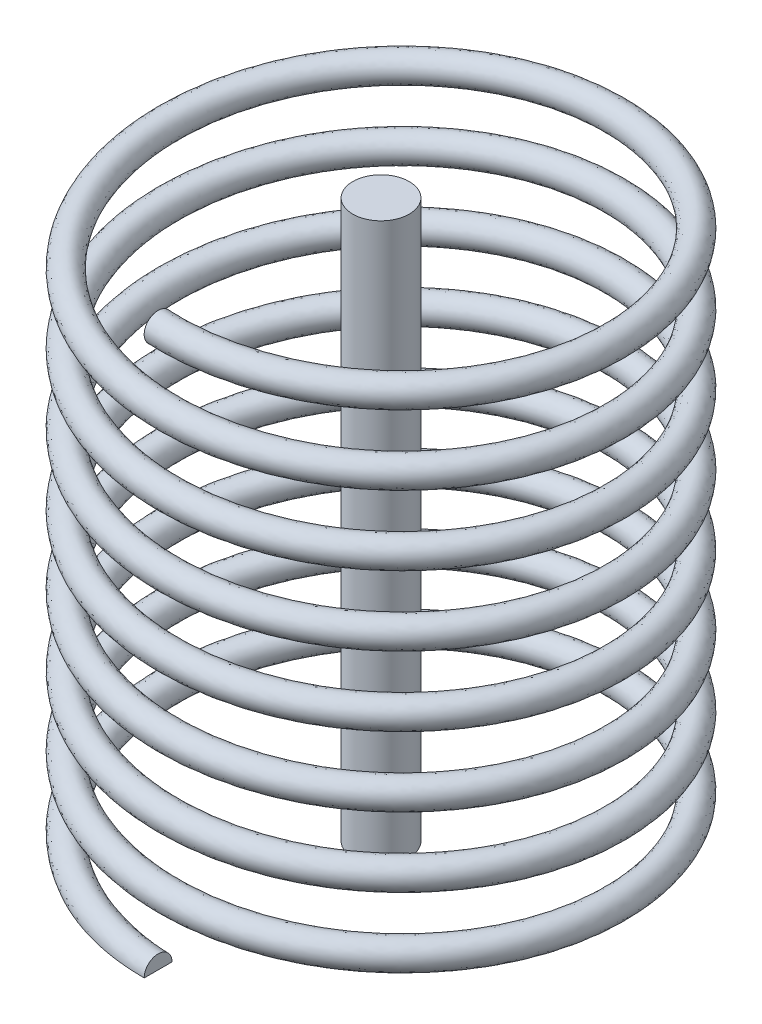
SolidWorks part; units mm, degrees
ref_plane "前视" through (0, 0, 0) normal (0, 0, 1) x (1, 0, 0)
ref_plane "上视" through (0, 0, 0) normal (0, 1, 0) x (1, 0, 0)
ref_plane "右视" through (0, 0, 0) normal (1, 0, 0) x (0, 0, -1)
sketch "草图2" plane through (0, 0, 0) normal (0, 1, 0) x (1, 0, 0)
  circle A0 centre (0, 0) radius 4
  dimension "D1" = 8
curve "螺旋线/涡状线1" pitch 1.25 height 10 turns 8
sketch "草图3" plane through (0, 0, 0) normal (1, 0, 0) x (0, 0, -1)
  line L0 (0, 0) -> (-4, 0) construction
  circle A0 centre (-4, 0) radius 0.25
  spline S0 degree 3 poles (-4, 0) (-4, 0.0259) (-3.7917, 0.0782) (-2.9021, 0.1562) (-1.5706, 0.2344) (0, 0.3125) (1.5706, 0.3906) (2.9021, 0.4687) (3.7917, 0.5469) (4.1041, 0.625) (3.7917, 0.7031) (2.9021, 0.7812) (1.5706, 0.8594) (0, 0.9375) (-1.5706, 1.0156) (-2.9021, 1.0937) (-3.7917, 1.1719) (-4.1041, 1.25) (-3.7917, 1.3281) (-2.9021, 1.4062) (-1.5706, 1.4844) (0, 1.5625) (1.5706, 1.6406) (2.9021, 1.7188) (3.7917, 1.7969) (4.1041, 1.875) (3.7917, 1.9531) (2.9021, 2.0313) (1.5706, 2.1094) (0, 2.1875) (-1.5706, 2.2656) (-2.9021, 2.3438) (-3.7917, 2.4219) (-4.1041, 2.5) (-3.7917, 2.5781) (-2.9021, 2.6562) (-1.5706, 2.7344) (0, 2.8125) (1.5706, 2.8906) (2.9021, 2.9688) (3.7917, 3.0469) (4.1041, 3.125) (3.7917, 3.2031) (2.9021, 3.2813) (1.5706, 3.3594) (0, 3.4375) (-1.5706, 3.5156) (-2.9021, 3.5938) (-3.7917, 3.6719) (-4.1041, 3.75) (-3.7917, 3.8281) (-2.9021, 3.9063) (-1.5706, 3.9844) (0, 4.0625) (1.5706, 4.1406) (2.9021, 4.2188) (3.7917, 4.2969) (4.1041, 4.375) (3.7917, 4.4531) (2.9021, 4.5313) (1.5706, 4.6094) (0, 4.6875) (-1.5706, 4.7656) (-2.9021, 4.8438) (-3.7917, 4.9219) (-4.1041, 5) (-3.7917, 5.0781) (-2.9021, 5.1563) (-1.5706, 5.2344) (0, 5.3125) (1.5706, 5.3906) (2.9021, 5.4688) (3.7917, 5.5469) (4.1041, 5.625) (3.7917, 5.7031) (2.9021, 5.7813) (1.5706, 5.8594) (0, 5.9375) (-1.5706, 6.0156) (-2.9021, 6.0938) (-3.7917, 6.1719) (-4.1041, 6.25) (-3.7917, 6.3281) (-2.9021, 6.4063) (-1.5706, 6.4844) (0, 6.5625) (1.5706, 6.6406) (2.9021, 6.7188) (3.7917, 6.7969) (4.1041, 6.875) (3.7917, 6.9531) (2.9021, 7.0313) (1.5706, 7.1094) (0, 7.1875) (-1.5706, 7.2656) (-2.9021, 7.3438) (-3.7917, 7.4219) (-4.1041, 7.5) (-3.7917, 7.5781) (-2.9021, 7.6563) (-1.5706, 7.7344) (0, 7.8125) (1.5706, 7.8906) (2.9021, 7.9688) (3.7917, 8.0469) (4.1041, 8.125) (3.7917, 8.2031) (2.9021, 8.2813) (1.5706, 8.3594) (0, 8.4375) (-1.5706, 8.5156) (-2.9021, 8.5938) (-3.7917, 8.6719) (-4.1041, 8.75) (-3.7917, 8.8281) (-2.9021, 8.9063) (-1.5706, 8.9844) (0, 9.0625) (1.5706, 9.1406) (2.9021, 9.2188) (3.7917, 9.2969) (4.1041, 9.375) (3.7917, 9.4531) (2.9021, 9.5313) (1.5706, 9.6094) (0, 9.6875) (-1.5706, 9.7656) (-2.9021, 9.8438) (-3.7917, 9.9218) (-4, 9.9741) (-4, 10) knots 0 0 0 0 0.007812 0.015625 0.023437 0.03125 0.039062 0.046875 0.054687 0.0625 0.070312 0.078125 0.085937 0.09375 0.101562 0.109375 0.117187 0.125 0.132812 0.140625 0.148437 0.15625 0.164062 0.171875 0.179687 0.1875 0.195312 0.203125 0.210937 0.21875 0.226562 0.234375 0.242187 0.25 0.257812 0.265625 0.273437 0.28125 0.289062 0.296875 0.304687 0.3125 0.320312 0.328125 0.335937 0.34375 0.351562 0.359375 0.367187 0.375 0.382812 0.390625 0.398437 0.40625 0.414062 0.421875 0.429687 0.4375 0.445312 0.453125 0.460937 0.46875 0.476562 0.484375 0.492187 0.5 0.507812 0.515625 0.523437 0.53125 0.539062 0.546875 0.554687 0.5625 0.570312 0.578125 0.585937 0.59375 0.601562 0.609375 0.617187 0.625 0.632812 0.640625 0.648437 0.65625 0.664062 0.671875 0.679687 0.6875 0.695312 0.703125 0.710937 0.71875 0.726562 0.734375 0.742187 0.75 0.757812 0.765625 0.773437 0.78125 0.789062 0.796875 0.804687 0.8125 0.820312 0.828125 0.835937 0.84375 0.851562 0.859375 0.867187 0.875 0.882812 0.890625 0.898437 0.90625 0.914062 0.921875 0.929687 0.9375 0.945312 0.953125 0.960937 0.96875 0.976562 0.984375 0.992187 1 1 1 1 construction
  dimension "D1" = 0.5
sweep "扫描1" add profiles "草图3" path "螺旋线/涡状线1"
sketch "草图4" plane through (0, 0, 0) normal (0, 1, 0) x (1, 0, 0)
  circle A0 centre (0, 0) radius 5.626
extrude "切除-拉伸1" cut sketch "草图4" against normal blind 10
sketch "草图5" plane through (0, 0, 0) normal (0, -1, 0) x (1, 0, 0)
  circle A0 centre (0, 0) radius 0.5066
extrude "凸台-拉伸1" add sketch "草图5" against normal blind 10 separate body
